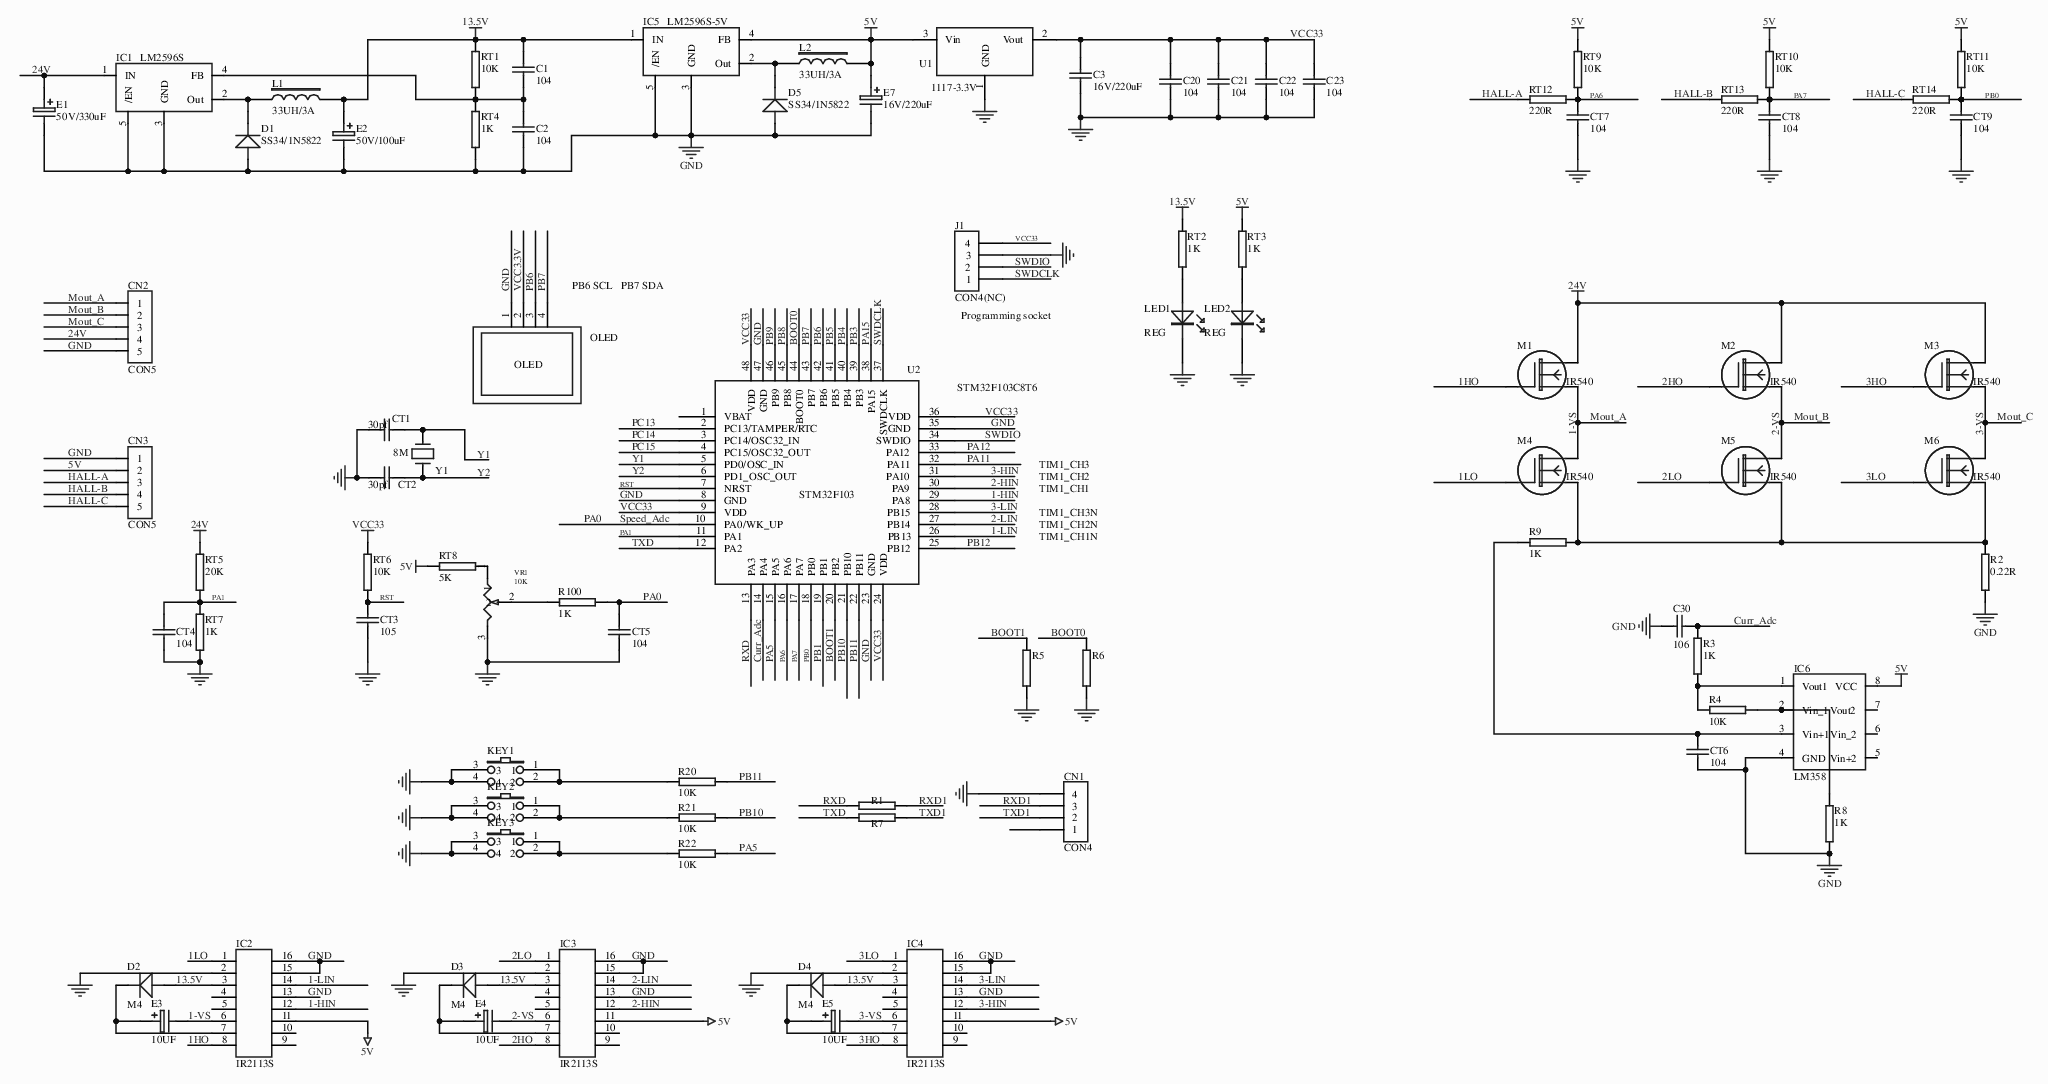
[diagram p0: MISC58867-3.schdoc]
# Altium project MISC58867-2.PrjPcb
1 sheet, 83 parts. Net scope: global (net labels, ports and power ports of the same name join across sheets).
Board file: MISC58867.pcbdoc

## Sheet MISC58867-3.schdoc
size 566 x 399 mm; Name: MISC58867

### Parts
C1  104  [C0603]
C2  104  [C0603]
C3  16V/220uF  [CAP-TH_BD5.0-P2.00-D0.8-FD-10UF50VC110GL]
C20  104  [C0603]
C21  104  [C0603]
C22  104  [C0603]
C23  104  [C0603]
C30  106  [CAP-TH_BD5.0-P2.00-D0.8-FD-10UF50VC110GL]
CN1  CON4  [CON4]
CN2  CON5  [CON5]
CN3  CON5  [CON5]
CT1  30pf  [C0603]
CT2  30pf  [C0603]
CT3  105  [C0603]
CT4  104  [C0603]
CT5  104  [C0603]
CT6  104  [C0603]
CT7  104  [C0603]
CT8  104  [C0603]
CT9  104  [C0603]
D1  SS34/1N5822  [SMA_L4.3-W2.5-LS5.0-RD]
D2  M4  [SMA_L4.3-W2.5-LS5.0-RD]
D3  M4  [SMA_L4.3-W2.5-LS5.0-RD]
D4  M4  [SMA_L4.3-W2.5-LS5.0-RD]
D5  SS34/1N5822  [SMA_L4.3-W2.5-LS5.0-RD]
E1  50V/330uF  [50v/330uf]
E2  50V/100uF  [50V/100UF]
E3  10UF  [CAP-TH_BD5.0-P2.00-D0.8-FD-10UF50VC110GL]
E4  10UF  [CAP-TH_BD5.0-P2.00-D0.8-FD-10UF50VC110GL]
E5  10UF  [CAP-TH_BD5.0-P2.00-D0.8-FD-10UF50VC110GL]
E7  16V/220uF  [16V/220UF]
IC1  LM2596S  [LM2596S]
IC2  IR2113S  [SOP-16]
IC3  IR2113S  [SOP-16]
IC4  IR2113S  [SOP-16]
IC5  LM2596S-5V  [LM2596S]
IC6  LM358  [lm358]
J1  CON4(NC)  [HDR-TH_4P-P2.54-V-F]
KEY1  (no value)  [SW-PB1]
KEY2  (no value)  [SW-PB1]
KEY3  (no value)  [SW-PB1]
L1  33UH/3A  [IND-SMD_L11.5-W10.5_MWSA1004]
L2  33UH/3A  [IND-SMD_L11.5-W10.5_MWSA1004]
LED1  REG  [LED0603]
LED2  REG  [LED0603]
M1  IR540  [IR5401]
M2  IR540  [IR5401]
M3  IR540  [IR5401]
M4  IR540  [IR5401]
M5  IR540  [IR5401]
M6  IR540  [IR5401]
OLED  OLED  [OLED]  (value not drawn)
R1  100R  [R0603]  (value not drawn)
R2  0.22R  [R0603]
R3  1K  [R0603]
R4  10K  [R0603]
R5  4.7K  [R0603]  (value not drawn)
R6  4.7K  [R0603]  (value not drawn)
R7  100R  [R0603]  (value not drawn)
R8  1K  [R0603]
R9  1K  [R0603]
R20  10K  [R0603]
R21  10K  [R0603]
R22  10K  [R0603]
R100  1K  [R0603]
RT1  10K  [R0603]
RT2  1K  [R0603]
RT3  1K  [R0603]
RT4  1K  [R0603]
RT5  20K  [R0603]
RT6  10K  [R0603]
RT7  1K  [R0603]
RT8  5K  [R0603]
RT9  10K  [R0603]
RT10  10K  [R0603]
RT11  10K  [R0603]
RT12  220R  [R0603]
RT13  220R  [R0603]
RT14  220R  [R0603]
U1  1117-3.3V  [1117-3.3V]
U2  STM32F103C8T6  [STM32F103C8T6]
VR1  10K  [R_3296]
Y1  8M  [HC-49S_L11.5-W5.0-P4.88]

### Nets
5V: CN3.2 E7.1 IC2.11 IC3.11 IC4.11 IC5.4(FB) IC6.8(VCC) L2.2 RT3.2 RT8.2 RT9.2 RT10.2 RT11.2 U1.3(Vin)
13.5V: C1.1 D2.2(A) D3.2(A) D4.2(A) E2.1 IC2.3 IC3.3 IC4.3 IC5.1(IN) L1.2 RT1.2 RT2.2
24V: CN2.4 E1.1 IC1.1(IN) M1.2 M2.2 M3.2 RT5.2
GND: C2.2 C3.2 C20.2 C21.2 C22.2 C23.2 C30.2 CN2.5 CN3.1 CT1.2 CT2.1 CT3.1 CT4.1 CT5.1 CT6.1 CT7.1 CT8.1 CT9.1 D1.2(A) D5.2(A) E1.2 E2.2 E7.2 IC1.3(GND) IC1.5(/EN) IC2.2 IC2.13 IC2.15 IC2.16 IC3.2 IC3.13 IC3.15 IC3.16 IC4.2 IC4.13 IC4.15 IC4.16 IC5.3(GND) IC5.5(/EN) IC6.4(GND) J1.3 KEY1.3 KEY1.4 KEY2.3 KEY2.4 KEY3.3 KEY3.4 LED1.2 LED2.2 OLED.1 R2.2 R5.1 R6.1 R8.2 RT4.1 RT7.1 U1.1(GND) U2.8(GND) U2.23(GND) U2.35(GND) U2.47(GND) VR1.3
VCC: CN1.4
VCC33: C3.1 C20.1 C21.1 C22.1 C23.1 J1.4 RT6.2 U1.2(Vout) U2.9(VDD) U2.24(VDD) U2.36(VDD) U2.48(VDD)
1-HIN: IC2.12 U2.29(PA8)
1-LIN: IC2.14 U2.26(PB13)
1-VS: CN2.1 E3.2 IC2.6 M1.3 M4.2  [also labelled Mout_A]
1HO: IC2.8 M1.1
1LO: IC2.1 M4.1
2-HIN: IC3.12 U2.30(PA9)
2-LIN: IC3.14 U2.27(PB14)
2-VS: CN2.2 E4.2 IC3.6 M2.3 M5.2  [also labelled Mout_B]
2HO: IC3.8 M2.1
2LO: IC3.1 M5.1
3-HIN: IC4.12 U2.31(PA10)
3-LIN: IC4.14 U2.28(PB15)
3-VS: CN2.3 E5.2 IC4.6 M3.3 M6.2  [also labelled Mout_C]
3HO: IC4.8 M3.1
3LO: IC4.1 M6.1
BOOT0: R6.2 U2.44(BOOT0)
BOOT1: R5.2 U2.20(PB2)
Curr_Adc: C30.1 R3.1 U2.14(PA4)
HALL-A: CN3.3 RT12.2
HALL-B: CN3.4 RT13.2
HALL-C: CN3.5 RT14.2
PA0: CT5.2 R100.1 U2.10(PA0/WK_UP)  [also labelled Speed_Adc]
PA1: CT4.2 RT5.1 RT7.2 U2.11(PA1)
PA5: R22.1 U2.15(PA5)
PA6: CT7.2 RT9.1 RT12.1 U2.16(PA6)
PA7: CT8.2 RT10.1 RT13.1 U2.17(PA7)
PA11: U2.32(PA11)
PA12: U2.33(PA12)
PA15: U2.38(PA15)
PB0: CT9.2 RT11.1 RT14.1 U2.18(PB0)
PB1: U2.19(PB1)
PB3: U2.39(PB3)
PB4: U2.40(PB4)
PB5: U2.41(PB5)
PB6: OLED.3 U2.42(PB6)
PB7: OLED.4 U2.43(PB7)
PB8: U2.45(PB8)
PB9: U2.46(PB9)
PB10: R21.1 U2.21(PB10)
PB11: R20.1 U2.22(PB11)
PB12: U2.25(PB12)
PC13: U2.2(PC13/TAMPER/RTC)
PC14: U2.3(PC14/OSC32_IN)
PC15: U2.4(PC15/OSC32_OUT)
RST: CT3.2 RT6.1 U2.7(NRST)
RXD: R1.2 U2.13(PA3)
RXD1: CN1.3 R1.1
SWDCLK: J1.1 U2.37(SWDCLK)
SWDIO: J1.2 U2.34(SWDIO)
TXD: R7.2 U2.12(PA2)
TXD1: CN1.2 R7.1
VCC3.3V: OLED.2
Y1: CT1.1 U2.5(PD0/OSC_IN) Y1.2
Y2: CT2.2 U2.6(PD1_OSC_OUT) Y1.1
NetC1_2: C1.2 C2.1 IC1.4(FB) RT1.1 RT4.2
NetCT6_2: CT6.2 IC6.3(Vin+1) R9.2
NetD1_1: D1.1(K) IC1.2(Out) L1.1
NetD2_1: D2.1(K) E3.1 IC2.7
NetD3_1: D3.1(K) E4.1 IC3.7
NetD4_1: D4.1(K) E5.1 IC4.7
NetD5_1: D5.1(K) IC5.2(Out) L2.1
NetIC6_1: IC6.1(Vout1) R3.2 R4.2
NetIC6_2: IC6.2(Vin_1) R4.1 R8.1
NetKEY1_1: KEY1.1 KEY1.2 R20.2
NetKEY2_1: KEY2.1 KEY2.2 R21.2
NetKEY3_1: KEY3.1 KEY3.2 R22.2
NetLED1_1: LED1.1 RT2.1
NetLED2_1: LED2.1 RT3.1
NetM4_3: M4.3 M5.3 M6.3 R2.1 R9.1
NetR100_2: R100.2 VR1.2
NetRT8_1: RT8.1 VR1.1

Not connected (* = marked no-connect by the designer): CN1 1; IC2 4* 5* 9* 10*; IC3 4* 5* 9* 10*; IC4 4* 5* 9* 10*; IC6 5(Vin+2) 6(Vin_2) 7(Vout2); U2 1(VBAT)

### Notes on the sheet
- (near OLED) PB6 SCL   PB7 SDA
- (near J1) Programming socket
- TIM1_CH3
- TIM1_CH2N
- TIM1_CH3N
- TIM1_CH1
- TIM1_CH2
- TIM1_CH1N

### Library data of the parts
C1 = CAP: Capacitor; Origin Footprint: C-0603; OriginFootprint 3: C0603X; UniqueId: b4693cfd16d534cd; AddInBom: yes; Device: CAP; OriginFootprint 2: C0603; DesignItemID: CAP; LibraryName: *; SymbolName: CAP
C2 = CAP: Capacitor; Origin Footprint: C-0603; OriginFootprint 3: C0603X; UniqueId: a2c5d49bc5dde298; AddInBom: yes; Device: CAP; OriginFootprint 2: C0603; DesignItemID: CAP; LibraryName: *; SymbolName: CAP
C3 = CAP: Capacitor; Origin Footprint: CD50MS-6355; OriginFootprint 2: C0603; OriginFootprint 3: C0603X; UniqueId: cc82bf2c2e22e605; AddInBom: yes; Device: CAP; DesignItemID: CAP; LibraryName: *; SymbolName: CAP
C20 = CAP: Capacitor; Origin Footprint: C-0603; OriginFootprint 3: C0603X; UniqueId: 97d7532320e593d5; AddInBom: yes; Device: CAP; OriginFootprint 2: C0603; DesignItemID: CAP; LibraryName: *; SymbolName: CAP
C21 = CAP: Capacitor; Origin Footprint: C-0603; OriginFootprint 3: C0603X; UniqueId: 0259cc883dd91c7a; AddInBom: yes; Device: CAP; OriginFootprint 2: C0603; DesignItemID: CAP; LibraryName: *; SymbolName: CAP
C22 = CAP: Capacitor; Origin Footprint: C-0603; OriginFootprint 3: C0603X; UniqueId: 7f35450ac3171d20; AddInBom: yes; Device: CAP; OriginFootprint 2: C0603; DesignItemID: CAP; LibraryName: *; SymbolName: CAP
C23 = CAP: Capacitor; Origin Footprint: C-0603; OriginFootprint 3: C0603X; UniqueId: 8bc5c1e1749a19fa; AddInBom: yes; Device: CAP; OriginFootprint 2: C0603; DesignItemID: CAP; LibraryName: *; SymbolName: CAP
C30 = CAP_3: Origin Footprint: C-0603; OriginFootprint 2: C0603X; UniqueId: a2ee6ceb65d30336; SymbolName: CAP; AddInBom: yes; Device: CAP_3; DesignItemID: CAP; LibraryName: *
CN1 = CON4_1: Connector; Origin Footprint: 4PIN 2.54; UniqueId: f8333110677ba079; AddInBom: yes; Device: CON4_1; DesignItemID: CON4; LibraryName: *; SymbolName: CON4
CN2 = CON5: Origin Footprint: KF301-5.0 - OK; UniqueId: b78ba3be0e9a0822; AddInBom: yes; Device: CON5; DesignItemID: CON5; LibraryName: 60-68-DYZJ-09; SymbolName: CON5
CN3 = CON5: Origin Footprint: KF301-5.0 - OK; UniqueId: 8e2184f8ebdd0e15; AddInBom: yes; Device: CON5; DesignItemID: CON5; LibraryName: 60-68-DYZJ-09; SymbolName: CON5
CT1 = CAP_2: Origin Footprint: C-0603; OriginFootprint 2: C0603X; UniqueId: 9c3083ceff059143; SymbolName: CAP; AddInBom: yes; Device: CAP_2; DesignItemID: CAP; LibraryName: *
CT2 = CAP_1: Origin Footprint: C-0603; OriginFootprint 2: C0603X; UniqueId: 97cd0ec21f247b41; SymbolName: CAP; AddInBom: yes; Device: CAP_1; DesignItemID: CAP; LibraryName: *
CT3 = CAP_1: Origin Footprint: C-0603; OriginFootprint 2: C0603X; UniqueId: b9424020e28cdfb7; SymbolName: CAP; AddInBom: yes; Device: CAP_1; DesignItemID: CAP; LibraryName: *
CT4 = CAP_1: Origin Footprint: C-0603; OriginFootprint 2: C0603X; UniqueId: e26874d26394bc5b; SymbolName: CAP; AddInBom: yes; Device: CAP_1; DesignItemID: CAP; LibraryName: *
CT5 = CAP_1: Origin Footprint: C-0603; OriginFootprint 2: C0603X; UniqueId: 64715565010f2323; SymbolName: CAP; AddInBom: yes; Device: CAP_1; DesignItemID: CAP; LibraryName: *
CT6 = CAP_1: Origin Footprint: C-0603; OriginFootprint 2: C0603X; UniqueId: 60d05169fb6ef2eb; SymbolName: CAP; AddInBom: yes; Device: CAP_1; DesignItemID: CAP; LibraryName: *
CT7 = CAP_1: Origin Footprint: C-0603; OriginFootprint 2: C0603X; UniqueId: 8817aa08e43946aa; SymbolName: CAP; AddInBom: yes; Device: CAP_1; DesignItemID: CAP; LibraryName: *
CT8 = CAP_1: Origin Footprint: C-0603; OriginFootprint 2: C0603X; UniqueId: 601b2546d846d1b4; SymbolName: CAP; AddInBom: yes; Device: CAP_1; DesignItemID: CAP; LibraryName: *
CT9 = CAP_1: Origin Footprint: C-0603; OriginFootprint 2: C0603X; UniqueId: 417a896e5fc6fb1b; SymbolName: CAP; AddInBom: yes; Device: CAP_1; DesignItemID: CAP; LibraryName: *
D1 = SS34/1N5822: Text Field1: 30; Text Field2: 20; Origin Footprint: SS34; UniqueId: 6eb2f7ba7a12821c; AddInBom: yes; Device: SS34/1N5822; DesignItemID: SS34/1N5822; LibraryName: SCH integrated library; SymbolName: SS34/1N5822; ConvertToPcb: yes
D2 = SS34/1N5822: Text Field1: 30; Text Field2: 20; Origin Footprint: SS34; UniqueId: cca08e5caf06c018; AddInBom: yes; Device: SS34/1N5822; DesignItemID: SS34/1N5822; LibraryName: SCH integrated library; SymbolName: SS34/1N5822; ConvertToPcb: yes
D3 = SS34/1N5822: Text Field1: 30; Text Field2: 20; Origin Footprint: SS34; UniqueId: 81689f1d3303caec; AddInBom: yes; Device: SS34/1N5822; DesignItemID: SS34/1N5822; LibraryName: SCH integrated library; SymbolName: SS34/1N5822; ConvertToPcb: yes
D4 = SS34/1N5822: Text Field1: 30; Text Field2: 20; Origin Footprint: SS34; UniqueId: 6a4368da87585c93; AddInBom: yes; Device: SS34/1N5822; DesignItemID: SS34/1N5822; LibraryName: SCH integrated library; SymbolName: SS34/1N5822; ConvertToPcb: yes
D5 = SS34/1N5822: Text Field1: 30; Text Field2: 20; Origin Footprint: SS34; UniqueId: aa27cf4c2f614704; AddInBom: yes; Device: SS34/1N5822; DesignItemID: SS34/1N5822; LibraryName: SCH integrated library; SymbolName: SS34/1N5822; ConvertToPcb: yes
E1 = ELECTRO1: Origin Footprint: EC3.5/8; UniqueId: b39237d7ae5e829b; AddInBom: yes; Device: ELECTRO1; DesignItemID: ELECTRO1; LibraryName: *; SymbolName: ELECTRO1
E2 = ELECTRO1: Origin Footprint: EC3.5/8; UniqueId: abef5cd3f8e4d13c; AddInBom: yes; Device: ELECTRO1; DesignItemID: ELECTRO1; LibraryName: *; SymbolName: ELECTRO1
E3 = ELECTRO1: Origin Footprint: C-1206; UniqueId: f188e0093434a5f2; AddInBom: yes; Device: ELECTRO1; DesignItemID: ELECTRO1; LibraryName: *; SymbolName: ELECTRO1
E4 = ELECTRO1_1: Origin Footprint: C-1206; UniqueId: 6aff208ae90c8695; AddInBom: yes; Device: ELECTRO1_1; DesignItemID: ELECTRO1; LibraryName: *; SymbolName: ELECTRO1
E5 = ELECTRO1_1: Origin Footprint: C-1206; UniqueId: 039ed5d04839b769; AddInBom: yes; Device: ELECTRO1_1; DesignItemID: ELECTRO1; LibraryName: *; SymbolName: ELECTRO1
E7 = ELECTRO1: Origin Footprint: CD50MS-6355; UniqueId: 865b013dd13d9ce3; AddInBom: yes; Device: ELECTRO1; DesignItemID: ELECTRO1; LibraryName: *; SymbolName: ELECTRO1
IC1 = LM2596S: Origin Footprint: TO263-5L; UniqueId: 0c396391978b946d; AddInBom: yes; Device: LM2596S; DesignItemID: LM2596S; LibraryName: Brushless motor; SymbolName: LM2596S
IC2 = SOP-16: UniqueId: 9c081cc57a023191; AddInBom: yes; Device: SOP-16; Origin Footprint: SOP-16; DesignItemID: SOP-16; LibraryName: *; SymbolName: SOP-16; FootprintName: SOP-16
IC3 = SOP-16: UniqueId: 0134910eb63ad9c7; AddInBom: yes; Device: SOP-16; Origin Footprint: SOP-16; DesignItemID: SOP-16; LibraryName: *; SymbolName: SOP-16; FootprintName: SOP-16
IC4 = SOP-16: UniqueId: 4c45a5f70a320848; AddInBom: yes; Device: SOP-16; Origin Footprint: SOP-16; DesignItemID: SOP-16; LibraryName: *; SymbolName: SOP-16; FootprintName: SOP-16
IC5 = LM2596S: Origin Footprint: TO263-5L; UniqueId: 5a160282001e4544; AddInBom: yes; Device: LM2596S; DesignItemID: LM2596S; LibraryName: Brushless motor; SymbolName: LM2596S
IC6 = HA17393: Origin Footprint: SO-8; UniqueId: 79b9ec0bc8d32cb6; AddInBom: yes; ModelId: 98770fc02da242c6bfad44f6a8da512b0819f05c4eef4c71ace90d822a990e87; Device: HA17393; DesignItemID: HA17393; LibraryName: *; SymbolName: HA17393; ModelName: SO-8
J1 = CON4: Connector; Origin Footprint: 4PIN 2.54; UniqueId: 51bfc0e5166a1c40; AddInBom: yes; Device: CON4; DesignItemID: CON4; LibraryName: *; SymbolName: CON4
KEY1 = SW-PB1: Origin Footprint: KEY-SMD 4; UniqueId: 3ea75fbfda3a0144; AddInBom: yes; Device: SW-PB1; DesignItemID: SW-PB1; LibraryName: *; SymbolName: SW-PB1
KEY2 = SW-PB1: Origin Footprint: KEY-SMD 4; UniqueId: f1e59420d253107b; AddInBom: yes; Device: SW-PB1; DesignItemID: SW-PB1; LibraryName: *; SymbolName: SW-PB1
KEY3 = SW-PB1: Origin Footprint: KEY-SMD 4; UniqueId: 3df087e0e8508ed7; AddInBom: yes; Device: SW-PB1; DesignItemID: SW-PB1; LibraryName: *; SymbolName: SW-PB1
L1 = INDUCTOR2: Origin Footprint: L12*12 - CD54; UniqueId: d450ceac7adb81c3; AddInBom: yes; Device: INDUCTOR2; DesignItemID: INDUCTOR2; LibraryName: *; SymbolName: INDUCTOR2
L2 = INDUCTOR2: Origin Footprint: L12*12 - CD54; UniqueId: 3f6ee2b1a34b017f; AddInBom: yes; Device: INDUCTOR2; DesignItemID: INDUCTOR2; LibraryName: *; SymbolName: INDUCTOR2
LED1 = LED: Origin Footprint: 0805-LED2; UniqueId: 7a65b453ee5a9ec2; AddInBom: yes; Device: LED; DesignItemID: LED; LibraryName: *; SymbolName: LED; ConvertToPcb: yes
LED2 = LED: Origin Footprint: 0805-LED2; UniqueId: 48c2d4982f4ec99a; AddInBom: yes; Device: LED; DesignItemID: LED; LibraryName: *; SymbolName: LED; ConvertToPcb: yes
M1 = MOSFET-N1_QDZ: Origin Footprint: TO263-NMOS; UniqueId: 20f64733a18c5380; AddInBom: yes; Device: MOSFET-N1_QDZ; DesignItemID: MOSFET-N1_QDZ; LibraryName: *; SymbolName: MOSFET-N1_QDZ
M2 = MOSFET-N1_QDZ: Origin Footprint: TO263-NMOS; UniqueId: 0b67e2366e5b1ba6; AddInBom: yes; Device: MOSFET-N1_QDZ; DesignItemID: MOSFET-N1_QDZ; LibraryName: *; SymbolName: MOSFET-N1_QDZ
M3 = MOSFET-N1_QDZ: Origin Footprint: TO263-NMOS; UniqueId: 4e48eb34ab40b298; AddInBom: yes; Device: MOSFET-N1_QDZ; DesignItemID: MOSFET-N1_QDZ; LibraryName: *; SymbolName: MOSFET-N1_QDZ
M4 = MOSFET-N1_QDZ: Origin Footprint: TO263-NMOS; UniqueId: 60a981ccfcd2d311; AddInBom: yes; Device: MOSFET-N1_QDZ; DesignItemID: MOSFET-N1_QDZ; LibraryName: *; SymbolName: MOSFET-N1_QDZ
M5 = MOSFET-N1_QDZ: Origin Footprint: TO263-NMOS; UniqueId: 6e34fdb5a2f89c68; AddInBom: yes; Device: MOSFET-N1_QDZ; DesignItemID: MOSFET-N1_QDZ; LibraryName: *; SymbolName: MOSFET-N1_QDZ
M6 = MOSFET-N1_QDZ: Origin Footprint: TO263-NMOS; UniqueId: 7a9c497156999796; AddInBom: yes; Device: MOSFET-N1_QDZ; DesignItemID: MOSFET-N1_QDZ; LibraryName: *; SymbolName: MOSFET-N1_QDZ
OLED = OLED: Origin Footprint: OLED I2C; AddInBom: yes; Symbol: OLED; Device: OLED; DesignItemID: OLED; LibraryName: SCH integrated library
R1 = RES2_3: UniqueId: 353b166cc2dee846; SymbolName: RES2; AddInBom: yes; ModelId: fc143cca1e79419f9cd78b61e9279f080819f05c4eef4c71ace90d822a990e87; Device: RES2_3; Origin Footprint: R0603; DesignItemID: RES2; LibraryName: *; FootprintName: R0603; ModelName: R0603
R2 = RES2_1: Origin Footprint: R15-1/2W; UniqueId: 6f63fc6711cfa315; SymbolName: RES2; AddInBom: yes; ModelId: fc143cca1e79419f9cd78b61e9279f080819f05c4eef4c71ace90d822a990e87; Device: RES2_1; DesignItemID: RES2; LibraryName: *; FootprintName: R0603; ModelName: R0603
R3 = RES2_1: UniqueId: fe89d0632cfce75f; SymbolName: RES2; AddInBom: yes; ModelId: fc143cca1e79419f9cd78b61e9279f080819f05c4eef4c71ace90d822a990e87; Device: RES2_1; Origin Footprint: R0603; DesignItemID: RES2; LibraryName: *; FootprintName: R0603; ModelName: R0603
R4 = RES2_1: UniqueId: fdc86a4b576d9e98; SymbolName: RES2; AddInBom: yes; ModelId: fc143cca1e79419f9cd78b61e9279f080819f05c4eef4c71ace90d822a990e87; Device: RES2_1; Origin Footprint: R0603; DesignItemID: RES2; LibraryName: *; FootprintName: R0603; ModelName: R0603
R5 = RES2_1: UniqueId: 9cdd622c9eeecfe7; SymbolName: RES2; AddInBom: yes; ModelId: fc143cca1e79419f9cd78b61e9279f080819f05c4eef4c71ace90d822a990e87; Device: RES2_1; Origin Footprint: R0603; DesignItemID: RES2; LibraryName: *; FootprintName: R0603; ModelName: R0603
R6 = RES2_1: UniqueId: e06ccd13940482ac; SymbolName: RES2; AddInBom: yes; ModelId: fc143cca1e79419f9cd78b61e9279f080819f05c4eef4c71ace90d822a990e87; Device: RES2_1; Origin Footprint: R0603; DesignItemID: RES2; LibraryName: *; FootprintName: R0603; ModelName: R0603
R7 = RES2_3: UniqueId: ba2c6d155e7fd301; SymbolName: RES2; AddInBom: yes; ModelId: fc143cca1e79419f9cd78b61e9279f080819f05c4eef4c71ace90d822a990e87; Device: RES2_3; Origin Footprint: R0603; DesignItemID: RES2; LibraryName: *; FootprintName: R0603; ModelName: R0603
R8 = RES2_1: UniqueId: 86d447fa2a9c8586; SymbolName: RES2; AddInBom: yes; ModelId: fc143cca1e79419f9cd78b61e9279f080819f05c4eef4c71ace90d822a990e87; Device: RES2_1; Origin Footprint: R0603; DesignItemID: RES2; LibraryName: *; FootprintName: R0603; ModelName: R0603
R9 = RES2_1: UniqueId: gge1; SymbolName: RES2; AddInBom: yes; ModelId: fc143cca1e79419f9cd78b61e9279f080819f05c4eef4c71ace90d822a990e87; Device: RES2_1; Origin Footprint: R0603; DesignItemID: RES2; LibraryName: *; FootprintName: R0603; ModelName: R0603
R20 = RES2_3: UniqueId: 13e77c54ede4b306; SymbolName: RES2; AddInBom: yes; ModelId: fc143cca1e79419f9cd78b61e9279f080819f05c4eef4c71ace90d822a990e87; Device: RES2_3; Origin Footprint: R0603; DesignItemID: RES2; LibraryName: *; FootprintName: R0603; ModelName: R0603
R21 = RES2_3: UniqueId: c77b08197b178948; SymbolName: RES2; AddInBom: yes; ModelId: fc143cca1e79419f9cd78b61e9279f080819f05c4eef4c71ace90d822a990e87; Device: RES2_3; Origin Footprint: R0603; DesignItemID: RES2; LibraryName: *; FootprintName: R0603; ModelName: R0603
R22 = RES2_3: UniqueId: fa394caafc8878d8; SymbolName: RES2; AddInBom: yes; ModelId: fc143cca1e79419f9cd78b61e9279f080819f05c4eef4c71ace90d822a990e87; Device: RES2_3; Origin Footprint: R0603; DesignItemID: RES2; LibraryName: *; FootprintName: R0603; ModelName: R0603
R100 = RES2_3: UniqueId: 150441bc09c68155; SymbolName: RES2; AddInBom: yes; ModelId: fc143cca1e79419f9cd78b61e9279f080819f05c4eef4c71ace90d822a990e87; Device: RES2_3; Origin Footprint: R0603; DesignItemID: RES2; LibraryName: *; FootprintName: R0603; ModelName: R0603
RT1 = RES2: UniqueId: 4cb6e3512c2d161f; AddInBom: yes; ModelId: fc143cca1e79419f9cd78b61e9279f080819f05c4eef4c71ace90d822a990e87; Device: RES2; Origin Footprint: R0603; DesignItemID: RES2; LibraryName: *; SymbolName: RES2; FootprintName: R0603; ModelName: R0603
RT2 = RES2: UniqueId: 30525bc082e97a7b; AddInBom: yes; ModelId: fc143cca1e79419f9cd78b61e9279f080819f05c4eef4c71ace90d822a990e87; Device: RES2; Origin Footprint: R0603; DesignItemID: RES2; LibraryName: *; SymbolName: RES2; FootprintName: R0603; ModelName: R0603
RT3 = RES2: UniqueId: f297941c1e519e1f; AddInBom: yes; ModelId: fc143cca1e79419f9cd78b61e9279f080819f05c4eef4c71ace90d822a990e87; Device: RES2; Origin Footprint: R0603; DesignItemID: RES2; LibraryName: *; SymbolName: RES2; FootprintName: R0603; ModelName: R0603
RT4 = RES2: UniqueId: 8789eddf6ab9f9d9; AddInBom: yes; ModelId: fc143cca1e79419f9cd78b61e9279f080819f05c4eef4c71ace90d822a990e87; Device: RES2; Origin Footprint: R0603; DesignItemID: RES2; LibraryName: *; SymbolName: RES2; FootprintName: R0603; ModelName: R0603
RT5 = RES2: UniqueId: 118d03610cace6fb; AddInBom: yes; ModelId: fc143cca1e79419f9cd78b61e9279f080819f05c4eef4c71ace90d822a990e87; Device: RES2; Origin Footprint: R0603; DesignItemID: RES2; LibraryName: *; SymbolName: RES2; FootprintName: R0603; ModelName: R0603
RT6 = RES2: UniqueId: 66ea078432e42e48; AddInBom: yes; ModelId: fc143cca1e79419f9cd78b61e9279f080819f05c4eef4c71ace90d822a990e87; Device: RES2; Origin Footprint: R0603; DesignItemID: RES2; LibraryName: *; SymbolName: RES2; FootprintName: R0603; ModelName: R0603
RT7 = RES2: UniqueId: 2e5e78d2b4b9f61d; AddInBom: yes; ModelId: fc143cca1e79419f9cd78b61e9279f080819f05c4eef4c71ace90d822a990e87; Device: RES2; Origin Footprint: R0603; DesignItemID: RES2; LibraryName: *; SymbolName: RES2; FootprintName: R0603; ModelName: R0603
RT8 = RES2_2: UniqueId: acda24587af66374; SymbolName: RES2; AddInBom: yes; ModelId: fc143cca1e79419f9cd78b61e9279f080819f05c4eef4c71ace90d822a990e87; Device: RES2_2; Origin Footprint: R0603; DesignItemID: RES2; LibraryName: *; FootprintName: R0603; ModelName: R0603
RT9 = RES2: UniqueId: 53db1d71a90a2820; AddInBom: yes; ModelId: fc143cca1e79419f9cd78b61e9279f080819f05c4eef4c71ace90d822a990e87; Device: RES2; Origin Footprint: R0603; DesignItemID: RES2; LibraryName: *; SymbolName: RES2; FootprintName: R0603; ModelName: R0603
RT10 = RES2: UniqueId: ff54964a25c2a640; AddInBom: yes; ModelId: fc143cca1e79419f9cd78b61e9279f080819f05c4eef4c71ace90d822a990e87; Device: RES2; Origin Footprint: R0603; DesignItemID: RES2; LibraryName: *; SymbolName: RES2; FootprintName: R0603; ModelName: R0603
RT11 = RES2: UniqueId: a9b79ae87fc797ae; AddInBom: yes; ModelId: fc143cca1e79419f9cd78b61e9279f080819f05c4eef4c71ace90d822a990e87; Device: RES2; Origin Footprint: R0603; DesignItemID: RES2; LibraryName: *; SymbolName: RES2; FootprintName: R0603; ModelName: R0603
RT12 = RES2_2: UniqueId: cbd91b8d2326ba56; SymbolName: RES2; AddInBom: yes; ModelId: fc143cca1e79419f9cd78b61e9279f080819f05c4eef4c71ace90d822a990e87; Device: RES2_2; Origin Footprint: R0603; DesignItemID: RES2; LibraryName: *; FootprintName: R0603; ModelName: R0603
RT13 = RES2_2: UniqueId: 3e07cdff4613ee8d; SymbolName: RES2; AddInBom: yes; ModelId: fc143cca1e79419f9cd78b61e9279f080819f05c4eef4c71ace90d822a990e87; Device: RES2_2; Origin Footprint: R0603; DesignItemID: RES2; LibraryName: *; FootprintName: R0603; ModelName: R0603
RT14 = RES2_2: UniqueId: 9cb7230009988d9e; SymbolName: RES2; AddInBom: yes; ModelId: fc143cca1e79419f9cd78b61e9279f080819f05c4eef4c71ace90d822a990e87; Device: RES2_2; Origin Footprint: R0603; DesignItemID: RES2; LibraryName: *; FootprintName: R0603; ModelName: R0603
U1 = 1117: Origin Footprint: 1117 3.3V TEST2; UniqueId: 1bdc0ab44f99f92d; AddInBom: yes; Device: 1117; DesignItemID: 1117; LibraryName: *; SymbolName: 1117
U2 = STM32F103C8T6: UniqueId: 48f0ae2437312dae; AddInBom: yes; Device: STM32F103C8T6; Origin Footprint: STM32F103C8T6; DesignItemID: STM32F103C8T6; LibraryName: *; SymbolName: STM32F103C8T6
VR1 = RES VAR 0932: Origin Footprint: 0932 potentiometer, vertical; UniqueId: 8e857b1cff8fa7ed; AddInBom: yes; Device: RES VAR 0932; DesignItemID: RES VAR 0932; LibraryName: SCH integrated library; SymbolName: RES VAR 0932
Y1 = CRYSTAL: Origin Footprint: XTL49-S-5032; UniqueId: 9790cc8ece124e27; AddInBom: yes; Device: CRYSTAL; DesignItemID: CRYSTAL; LibraryName: *; Description: Crystal; SymbolName: CRYSTAL